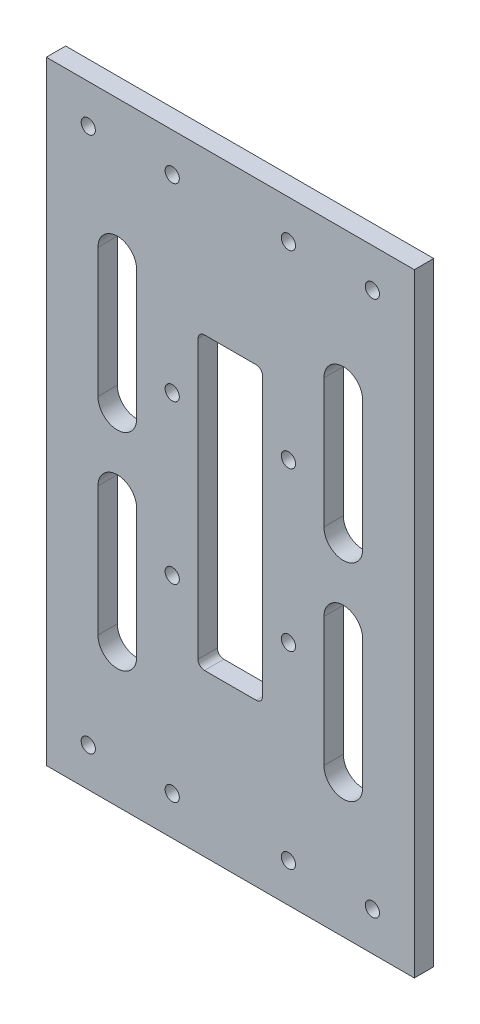
from build123d import *

# Parameters (mm, degrees)
SKETCH_1_W      = 570
SKETCH_1_H      = 950
SKETCH_1_R      = 11
EXTRUDE_1_DEPTH = 30


with BuildPart() as part:
    # 草图1 → 凸台-拉伸1 (new body)
    with BuildSketch(Plane.XY):
        with Locations((1800, 1250)):
            Rectangle(SKETCH_1_W, SKETCH_1_H)
        with Locations((1580, 1665)):
            Circle(SKETCH_1_R, mode=Mode.SUBTRACT)
        with Locations((1710, 1665)):
            Circle(SKETCH_1_R, mode=Mode.SUBTRACT)
        with Locations((1890, 1665)):
            Circle(SKETCH_1_R, mode=Mode.SUBTRACT)
        with Locations((2020, 1665)):
            Circle(SKETCH_1_R, mode=Mode.SUBTRACT)
        with Locations((1710, 1372.5)):
            Circle(SKETCH_1_R, mode=Mode.SUBTRACT)
        with Locations((1890, 1372.5)):
            Circle(SKETCH_1_R, mode=Mode.SUBTRACT)
        with Locations(Location((1710, 1127.5, 0), (0, 0, 180))):
            Circle(SKETCH_1_R, mode=Mode.SUBTRACT)
        with Locations(Location((1890, 1127.5, 0), (0, 0, 180))):
            Circle(SKETCH_1_R, mode=Mode.SUBTRACT)
        with Locations(Location((2020, 835, 0), (0, 0, 180))):
            Circle(SKETCH_1_R, mode=Mode.SUBTRACT)
        with Locations(Location((1890, 835, 0), (0, 0, 180))):
            Circle(SKETCH_1_R, mode=Mode.SUBTRACT)
        with Locations(Location((1710, 835, 0), (0, 0, 180))):
            Circle(SKETCH_1_R, mode=Mode.SUBTRACT)
        with Locations(Location((1580, 835, 0), (0, 0, 180))):
            Circle(SKETCH_1_R, mode=Mode.SUBTRACT)
        with BuildLine():
            Line((1840, 1025), (1760, 1025))
            ThreePointArc((1760, 1025), (1752.928932188, 1027.928932188), (1750, 1035))
            Line((1750, 1035), (1750, 1465))
            ThreePointArc((1750, 1465), (1752.928932188, 1472.071067812), (1760, 1475))
            Line((1760, 1475), (1840, 1475))
            ThreePointArc((1840, 1475), (1847.071067812, 1472.071067812), (1850, 1465))
            Line((1850, 1465), (1850, 1035))
            ThreePointArc((1850, 1035), (1847.071067812, 1027.928932188), (1840, 1025))
        make_face(mode=Mode.SUBTRACT)
        with BuildLine():
            Line((1655, 1510), (1655, 1310))
            ThreePointArc((1655, 1310), (1625, 1280), (1595, 1310))
            Line((1595, 1310), (1595, 1510))
            ThreePointArc((1595, 1510), (1625, 1540), (1655, 1510))
        make_face(mode=Mode.SUBTRACT)
        with BuildLine():
            Line((2005, 1510), (2005, 1310))
            ThreePointArc((2005, 1310), (1975, 1280), (1945, 1310))
            Line((1945, 1310), (1945, 1510))
            ThreePointArc((1945, 1510), (1975, 1540), (2005, 1510))
        make_face(mode=Mode.SUBTRACT)
        with BuildLine():
            Line((2005, 990), (2005, 1190))
            ThreePointArc((2005, 1190), (1975, 1220), (1945, 1190))
            Line((1945, 1190), (1945, 990))
            ThreePointArc((1945, 990), (1975, 960), (2005, 990))
        make_face(mode=Mode.SUBTRACT)
        with BuildLine():
            Line((1655, 990), (1655, 1190))
            ThreePointArc((1655, 1190), (1625, 1220), (1595, 1190))
            Line((1595, 1190), (1595, 990))
            ThreePointArc((1595, 990), (1625, 960), (1655, 990))
        make_face(mode=Mode.SUBTRACT)
    extrude(amount=EXTRUDE_1_DEPTH)


solid = part.part
